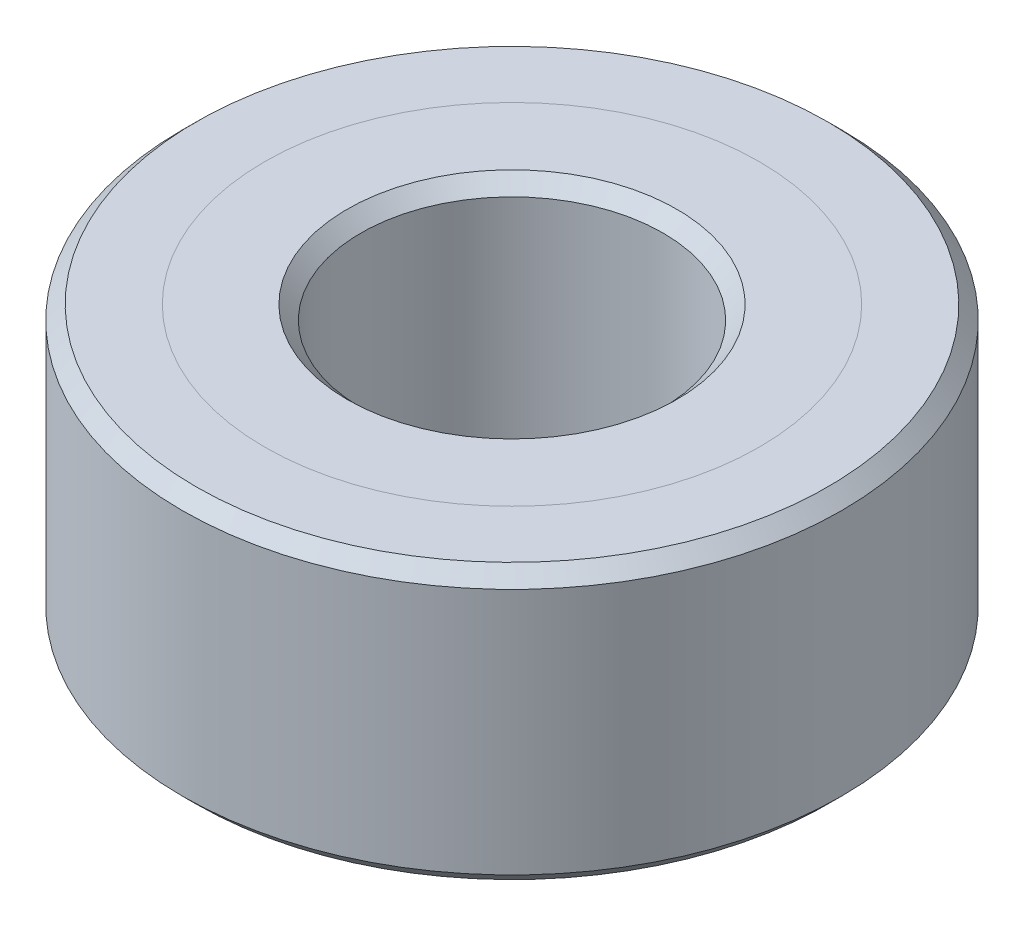
SolidWorks part; units mm, degrees
ref_plane "Front Plane" through (0, 0, 0) normal (0, 0, 1) x (1, 0, 0)
ref_plane "Top Plane" through (0, 0, 0) normal (0, 1, 0) x (1, 0, 0)
ref_plane "Right Plane" through (0, 0, 0) normal (1, 0, 0) x (0, 0, -1)
sketch "Sketch1" plane through (0, 0, 0) normal (0, 1, 0) x (1, 0, 0)
  circle A0 centre (0, 0) radius 15
  circle A1 centre (0, 0) radius 5.5
  dimension "D1" = 30
  dimension "D2" = 11
extrude "Boss-Extrude1" add sketch "Sketch1" along normal blind 10
chamfer "Chamfer1" distance 0.5 angle 45 2 edges at (0, 0, 15) (0, 10, 15)
sketch "Sketch2" plane through (0, 10, 0) normal (0, 1, 0) x (1, 0, 0)
  circle A0 centre (0, 0) radius 9
  circle A1 centre (0, 0) radius 15
  circle A2 centre (0, 0) radius 15 construction
  dimension "D1" = 18
extrude "Cut-Extrude1" cut sketch "Sketch2" against normal blind 10
sketch "Sketch3" plane through (0, 10, 0) normal (0, 1, 0) x (1, 0, 0)
  circle A0 centre (0, 0) radius 12
  circle A1 centre (0, 0) radius 9
  circle A2 centre (0, 0) radius 9 construction
  dimension "D1" = 24
extrude "Boss-Extrude2" add sketch "Sketch3" against normal up to surface (10 mm away) separate body up to face at (0, 0, 5.5)
chamfer "Chamfer2" distance 0.5 angle 45 2 edges at (0, 0, 12) (0, 10, 12)
chamfer "Chamfer3" distance 0.5 angle 45 2 edges at (0, 10, 5.5) (0, 0, 5.5)
